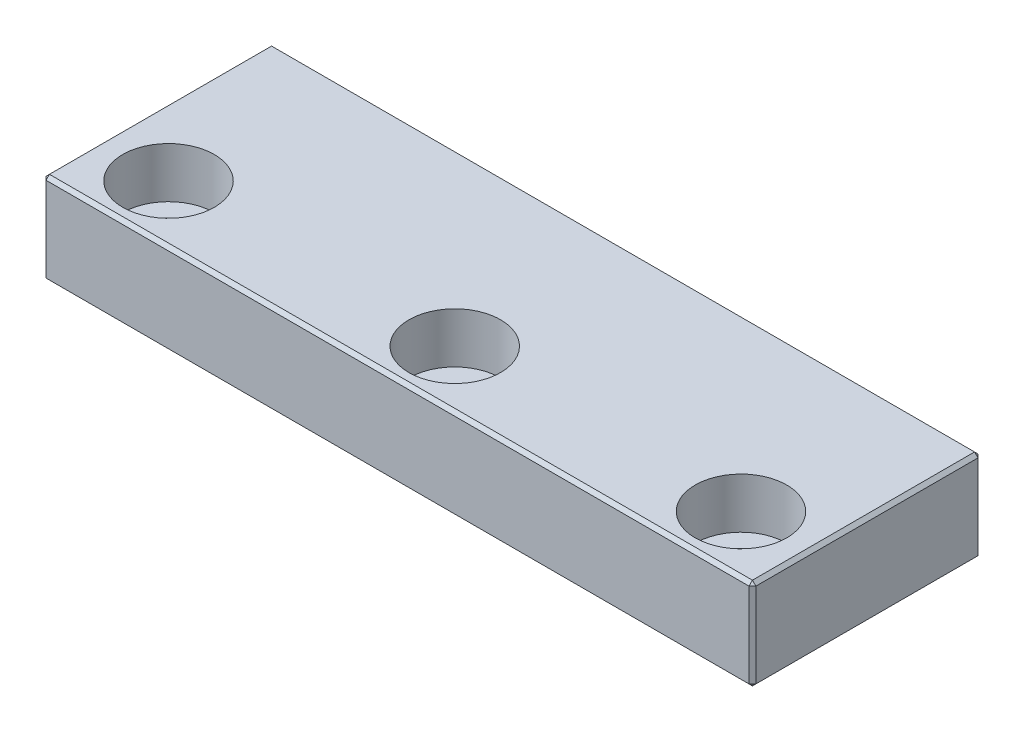
from build123d import *

# Parameters (mm, degrees)
SKETCH_1_W                   = 62
SKETCH_1_H                   = 20
EXTRUDE_1_DEPTH              = 8
HOLE_WIZARD_M4_1_D           = 4.5
HOLE_WIZARD_M4_1_CBORE_D     = 8
HOLE_WIZARD_M4_1_CBORE_DEPTH = 4.4
CHAMFER_1_SIZE               = 0.3


with BuildPart() as part:
    # 草图1 → 凸台-拉伸1 (new body)
    with BuildSketch(Plane(origin=(0, 0, 0), x_dir=(1, 0, 0), z_dir=(0, 1, 0))):
        Rectangle(SKETCH_1_W, SKETCH_1_H)
    extrude(amount=EXTRUDE_1_DEPTH)

    # M4 六角凹头螺钉的柱形沉头孔1 (through all)
    with Locations(Plane(origin=(0, 8, 0), x_dir=(1, 0, 0), z_dir=(0, 1, 0))):
        with Locations((-25, -5), (0, -5), (25, -5)):
            CounterBoreHole(HOLE_WIZARD_M4_1_D / 2, HOLE_WIZARD_M4_1_CBORE_D / 2, HOLE_WIZARD_M4_1_CBORE_DEPTH)

    # 倒角1
    chamfer_1_edges = [part.edges().sort_by_distance(p)[0] for p in [
        (-31, 8, 0),
        (0, 8, 10),
        (31, 8, 0),
        (0, 0, 10),
        (-31, 0, 0),
        (0, 0, -10),
        (31, 0, 0),
        (0, 8, -10),
        (31, 4, 10),
        (-31, 4, 10),
        (-31, 4, -10),
        (31, 4, -10),
    ]]
    chamfer(chamfer_1_edges, length=CHAMFER_1_SIZE)


solid = part.part
